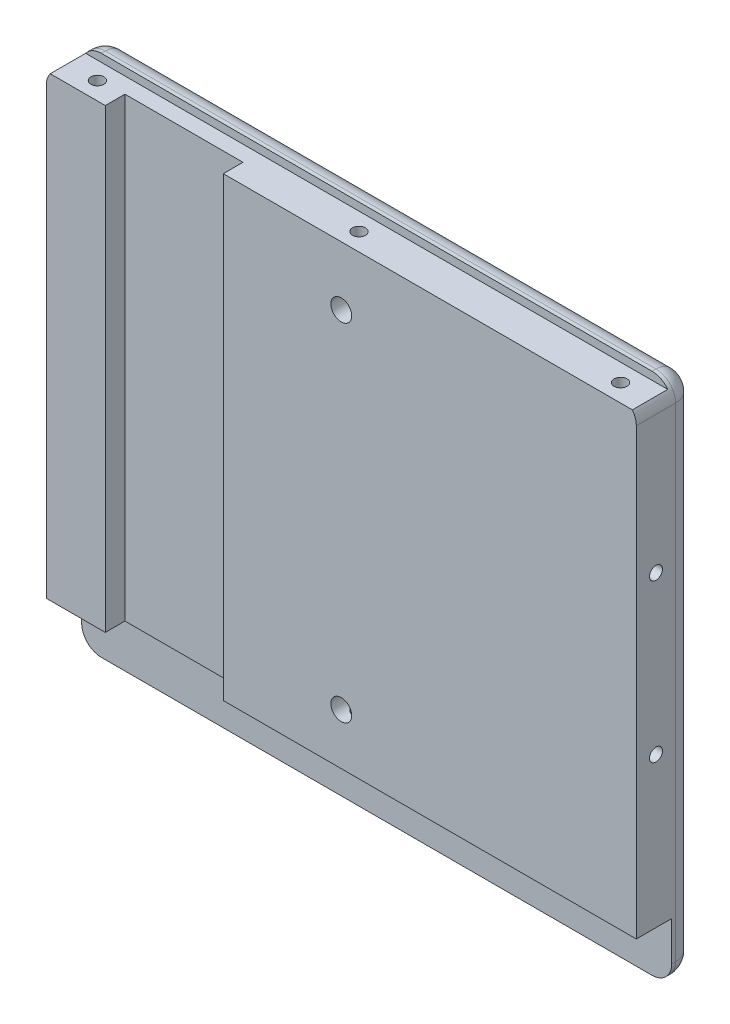
SolidWorks part; units mm, degrees
ref_plane "前视基准面" through (0, 0, 0) normal (0, 0, 1) x (1, 0, 0)
ref_plane "上视基准面" through (0, 0, 0) normal (0, 1, 0) x (1, 0, 0)
ref_plane "右视基准面" through (0, 0, 0) normal (1, 0, 0) x (0, 0, -1)
sketch "草图1" plane through (0, 0, 0) normal (0, 0, 1) x (1, 0, 0)
  line L1 (-75, 66.5) -> (75, 66.5)
  line L2 (-75, 66.5) -> (-75, -66.5)
  line L3 (-75, -66.5) -> (75, -66.5)
  line L4 (75, 66.5) -> (75, -66.5)
  line L5 (-75, 66.5) -> (75, -66.5) construction
  line L6 (-75, -66.5) -> (75, 66.5) construction
  point P0 (0, 0)
  dimension "D1" = 150
  dimension "D2" = 133
extrude "凸台-拉伸1" add sketch "草图1" along normal blind 15
sketch "草图2" plane through (75, 0, 0) normal (1, 0, 0) x (0, 0, -1)
  line L0 (-15, 66.5) -> (0, 66.5) construction
  line L1 (-38.5841, 92.8639) -> (-6, 92.8639)
  line L2 (-38.5841, 92.8639) -> (-38.5841, 64.5)
  line L3 (-38.5841, 64.5) -> (-6, 64.5)
  line L4 (-6, 92.8639) -> (-6, 64.5)
  line L5 (-38.5841, 92.8639) -> (-6, 64.5) construction
  line L6 (-38.5841, 64.5) -> (-6, 92.8639) construction
  line L7 (-15, -66.5) -> (-15, 66.5) construction
  point P0 (-22.292, 78.682)
  dimension "D1" = 2
  dimension "D2" = 9
extrude "切除-拉伸1" cut sketch "草图2" against normal through all
fillet "圆角8" radius 5 8 edges at (75, 66.5, 3) (-75, 66.5, 3) (-75, -66.5, 7.5) (75, -66.5, 7.5) (0, -66.5, 0) (-75, 0, 0) (75, 0, 0) (0, 66.5, 0)
hole_wizard "打孔尺寸(%根据)开槽圆柱头螺钉的类型1" positions "草图6" profile "草图5" counterbore size "M5" standard "GB" end condition through all
sketch "草图6" plane through (0, 0, 0) normal (0, 0, -1) x (-1, 0, 0)
  line L0 (-75, -61.5) -> (-75, 61.5) construction
  line L1 (-70, 66.5) -> (70, 66.5) construction
  line L2 (70, -66.5) -> (-70, -66.5) construction
  point P0 (0, 49.5)
  point P9 (0, -38.5)
  dimension "D1" = 75
  dimension "D2" = 17
  dimension "D3" = 28
sketch "草图5" plane through (0, 49.5, 0) normal (1, 0, 0) x (0, 1, 0)
  line L0 (0, 0) -> (0, 15)
  line L1 (0, 15) -> (2.65, 15)
  line L3 (2.65, 15) -> (2.65, 5.7)
  line L4 (2.65, 5.7) -> (5, 5.7)
  line L5 (5, 5.7) -> (5, 0)
  line L7 (5, 0) -> (0, 0)
  line L11 (0, -6.35) -> (0, 107.95) construction
  dimension "通孔孔直径" = 5.3
  dimension "通孔孔深度" = 15
  dimension "柱形沉头孔直径" = 10
  dimension "柱形沉头孔深度" = 5.7
hole_wizard "M4 螺纹孔3" positions "草图10" profile "草图9" tap size "M4" standard "GB"
sketch "草图10" plane through (0, 64.5, 0) normal (0, 1, 0) x (1, 0, 0)
  line L1 (-74, -15) -> (74, -15) construction
  line L3 (-66.5, -10.5) -> (66.5, -10.5) construction
  point P0 (0, -10.5)
  point P2 (66.5, -10.5)
  point P12 (-66.5, -10.5)
  dimension "D1" = 133
  dimension "D3" = 4.5
sketch "草图9" plane through (0, 64.5, 10.5) normal (1, 0, 0) x (0, 0, 1)
  line L0 (0, 0) -> (0, 16.4914)
  line L1 (0, 16.4914) -> (1.65, 15.5)
  line L2 (1.65, 15.5) -> (1.65, 0)
  line L5 (1.65, 0) -> (0, 0)
  line L10 (0, 16.4914) -> (-1.65, 15.5) construction
  line L11 (0, -6.35) -> (0, 107.95) construction
  dimension "螺纹孔钻头直径" = 3.3
  dimension "螺纹孔钻头深度" = 15.5
  dimension "导头角度" = 118
cosmetic thread "孔螺蚊线3" parameters "D1"=12, "D2"=4
cosmetic thread "孔螺蚊线4" parameters "D1"=12, "D2"=4
cosmetic thread "孔螺蚊线19" parameters "D1"=12, "D2"=4
sketch "草图20" plane through (0, -66.5, 0) normal (0, -1, 0) x (1, 0, 0)
  line L0 (-70, 15) -> (70, 15) construction
  line L1 (-314.4693, 145.1057) -> (117.2717, 145.1057)
  line L2 (-314.4693, 145.1057) -> (-314.4693, 6)
  line L3 (-314.4693, 6) -> (117.2717, 6)
  line L4 (117.2717, 145.1057) -> (117.2717, 6)
  line L5 (-314.4693, 145.1057) -> (117.2717, 6) construction
  line L6 (-314.4693, 6) -> (117.2717, 145.1057) construction
  point P0 (-98.5988, 75.5528)
  dimension "D1" = 9
extrude "切除-拉伸5" cut sketch "草图20" against normal blind 15
sketch "草图24" plane through (0, 0, 15) normal (0, 0, 1) x (1, 0, 0)
  line L1 (-60, 82.3999) -> (-30, 82.3999)
  line L2 (-60, 82.3999) -> (-60, -95.1031)
  line L3 (-60, -95.1031) -> (-30, -95.1031)
  line L4 (-30, 82.3999) -> (-30, -95.1031)
  line L5 (-60, 82.3999) -> (-30, -95.1031) construction
  line L6 (-60, -95.1031) -> (-30, 82.3999) construction
  line L7 (-75, 61.5) -> (-75, -51.5) construction
  point P0 (-45, -6.3516)
  dimension "D1" = 30
  dimension "D2" = 15
extrude "切除-拉伸6" cut sketch "草图24" against normal blind 5
hole_wizard "M4 螺纹孔2" positions "草图25" profile "草图26" tap size "M4" standard "GB"
sketch "草图25" plane through (0, -51.5, 0) normal (0, -1, 0) x (-1, 0, 0)
  line L0 (0, 0) -> (0, -51.4152) construction
  line L1 (30, -15) -> (-75, -15) construction
  point P18 (0, -10.5)
  point P20 (-66.5, -10.5)
  point P23 (66.5, -10.5)
  dimension "D1" = 133
  dimension "D2" = 4.5
sketch "草图26" plane through (-66.5, -51.5, 10.5) normal (1, 0, 0) x (0, 0, -1)
  line L0 (0, 0) -> (0, 12.4914)
  line L1 (0, 12.4914) -> (1.65, 11.5)
  line L2 (1.65, 11.5) -> (1.65, 0)
  line L5 (1.65, 0) -> (0, 0)
  line L10 (0, 12.4914) -> (-1.65, 11.5) construction
  line L11 (0, -6.35) -> (0, 107.95) construction
  dimension "螺纹孔钻头直径" = 3.3
  dimension "螺纹孔钻头深度" = 11.5
  dimension "导头角度" = 118
cosmetic thread "孔螺蚊线21" parameters "D1"=8, "D2"=4
cosmetic thread "孔螺蚊线22" parameters "D1"=8, "D2"=4
cosmetic thread "孔螺蚊线23" parameters "D1"=8, "D2"=4
hole_wizard "M4 螺纹孔1" positions "草图27" profile "草图28" tap size "M4" standard "GB"
sketch "草图27" plane through (75, 0, 0) normal (1, 0, 0) x (0, 0, -1)
  point P0 (-10, 26.6108)
  point P3 (-10, -13.3892)
sketch "草图28" plane through (75, 26.6108, 10) normal (0, 1, 0) x (0, 0, -1)
  line L0 (0, 0) -> (0, 12.9914)
  line L1 (0, 12.9914) -> (1.65, 12)
  line L2 (1.65, 12) -> (1.65, 0)
  line L5 (1.65, 0) -> (0, 0)
  line L10 (0, 12.9914) -> (-1.65, 12) construction
  line L11 (0, -6.35) -> (0, 107.95) construction
  dimension "螺纹孔钻头直径" = 3.3
  dimension "螺纹孔钻头深度" = 12
  dimension "导头角度" = 118
cosmetic thread "孔螺蚊线24" parameters "D1"=8, "D2"=4
cosmetic thread "孔螺蚊线25" parameters "D1"=8, "D2"=4
mirror "镜向1" about plane through (0, 0, 0) normal (1, 0, 0) of "M4 螺纹孔1"
